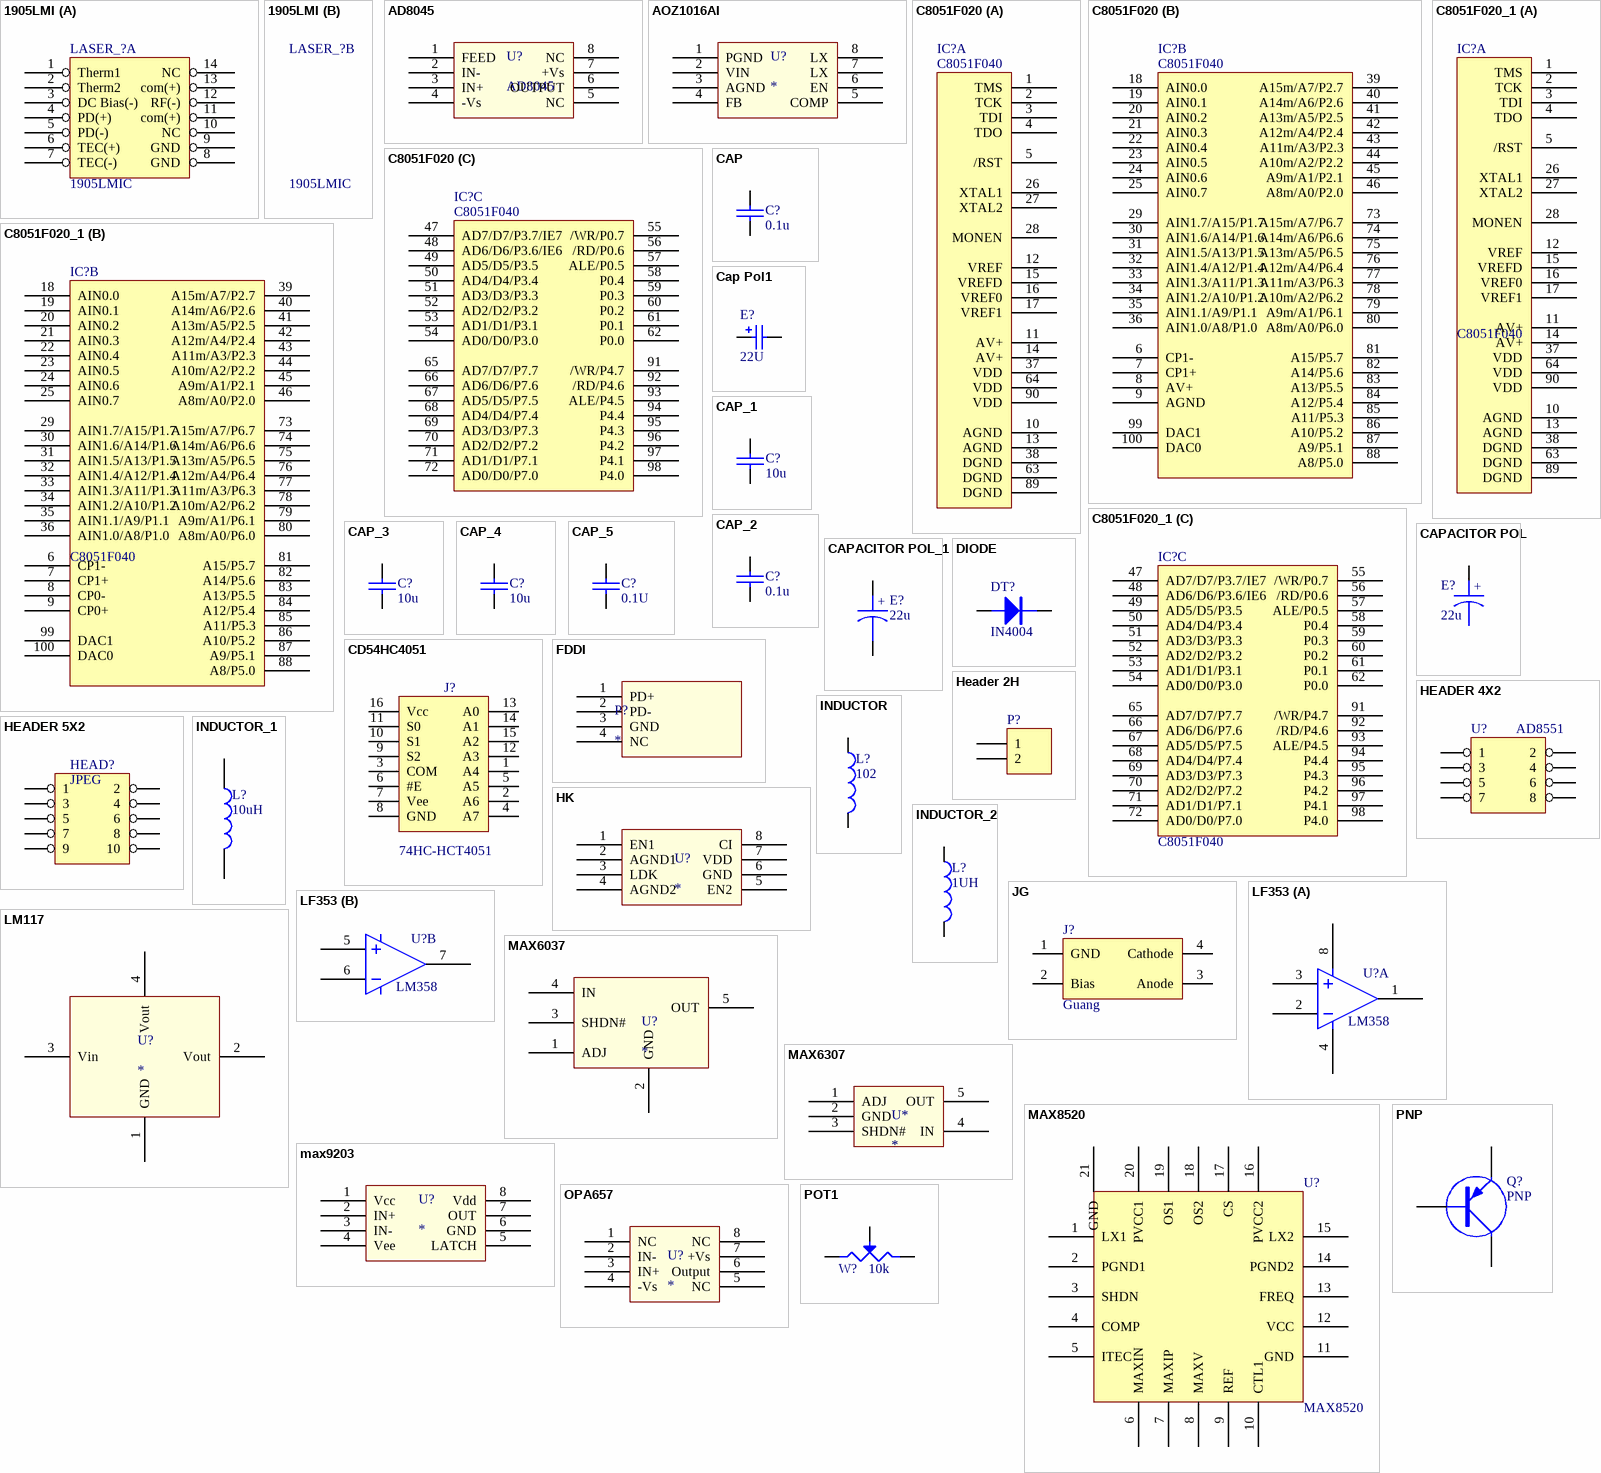
[diagram p0: symbols 1905LMI to POT1]
# Altium schematic symbol library MISC79012-5.SchLib: 47 symbols
Pins are listed as number, name and electrical type; pins without a type are passive.


## 1905LMI
designator LASER_?, comment 1905LMIC
Part Field 1: +5
footprint 1915LMM_LD
part A pins: 1 Therm1, 2 Therm2, 3 DC Bias(-), 4 PD(+), 5 PD(-), 6 TEC(+), 7 TEC(-), 8 GND, 9 GND, 10 NC, 11 com(+), 12 RF(-), 13 com(+), 14 NC

## AD8045
designator U?
pins: 1 FEED, 2 IN-, 3 IN+, 4 -Vs, 5 NC, 6 OUTPUT, 7 +Vs, 8 NC

## AOZ1016AI
designator U?
pins: 1 PGND, 2 VIN, 3 AGND, 4 FB, 5 COMP, 6 EN, 7 LX, 8 LX

## C8051F020
designator IC?, comment C8051F040
footprint TQFP100
part A pins: 1 TMS, 2 TCK, 3 TDI, 4 TDO, 5 /RST, 10 AGND, 11 AV+, 12 VREF, 13 AGND, 14 AV+, 15 VREFD, 16 VREF0, 17 VREF1, 26 XTAL1, 27 XTAL2, 28 MONEN, 37 VDD, 38 DGND, 63 DGND, 64 VDD, 89 DGND, 90 VDD
part B pins: 6 CP1-, 7 CP1+, 8 AV+, 9 AGND, 18 AIN0.0, 19 AIN0.1, 20 AIN0.2, 21 AIN0.3, 22 AIN0.4, 23 AIN0.5, 24 AIN0.6, 25 AIN0.7, 29 AIN1.7/A15/P1.7, 30 AIN1.6/A14/P1.6, 31 AIN1.5/A13/P1.5, 32 AIN1.4/A12/P1.4, 33 AIN1.3/A11/P1.3, 34 AIN1.2/A10/P1.2, 35 AIN1.1/A9/P1.1, 36 AIN1.0/A8/P1.0, 39 A15m/A7/P2.7, 40 A14m/A6/P2.6, 41 A13m/A5/P2.5, 42 A12m/A4/P2.4, 43 A11m/A3/P2.3, 44 A10m/A2/P2.2, 45 A9m/A1/P2.1, 46 A8m/A0/P2.0, 73 A15m/A7/P6.7, 74 A14m/A6/P6.6, 75 A13m/A5/P6.5, 76 A12m/A4/P6.4, 77 A11m/A3/P6.3, 78 A10m/A2/P6.2, 79 A9m/A1/P6.1, 80 A8m/A0/P6.0, 81 A15/P5.7, 82 A14/P5.6, 83 A13/P5.5, 84 A12/P5.4, 85 A11/P5.3, 86 A10/P5.2, 87 A9/P5.1, 88 A8/P5.0, 99 DAC1, 100 DAC0
part C pins: 47 AD7/D7/P3.7/IE7, 48 AD6/D6/P3.6/IE6, 49 AD5/D5/P3.5, 50 AD4/D4/P3.4, 51 AD3/D3/P3.3, 52 AD2/D2/P3.2, 53 AD1/D1/P3.1, 54 AD0/D0/P3.0, 55 /WR/P0.7, 56 /RD/P0.6, 57 ALE/P0.5, 58 P0.4, 59 P0.3, 60 P0.2, 61 P0.1, 62 P0.0, 65 AD7/D7/P7.7, 66 AD6/D6/P7.6, 67 AD5/D5/P7.5, 68 AD4/D4/P7.4, 69 AD3/D3/P7.3, 70 AD2/D2/P7.2, 71 AD1/D1/P7.1, 72 AD0/D0/P7.0, 91 /WR/P4.7, 92 /RD/P4.6, 93 ALE/P4.5, 94 P4.4, 95 P4.3, 96 P4.2, 97 P4.1, 98 P4.0
2 alternate drawings of the same symbol

## C8051F020_1
designator IC?, comment C8051F040
footprint TQFP100
part A pins: 1 TMS, 2 TCK, 3 TDI, 4 TDO, 5 /RST, 10 AGND, 11 AV+, 12 VREF, 13 AGND, 14 AV+, 15 VREFD, 16 VREF0, 17 VREF1, 26 XTAL1, 27 XTAL2, 28 MONEN, 37 VDD, 38 DGND, 63 DGND, 64 VDD, 89 DGND, 90 VDD
part B pins: 6 CP1-, 7 CP1+, 8 CP0-, 9 CP0+, 18 AIN0.0, 19 AIN0.1, 20 AIN0.2, 21 AIN0.3, 22 AIN0.4, 23 AIN0.5, 24 AIN0.6, 25 AIN0.7, 29 AIN1.7/A15/P1.7, 30 AIN1.6/A14/P1.6, 31 AIN1.5/A13/P1.5, 32 AIN1.4/A12/P1.4, 33 AIN1.3/A11/P1.3, 34 AIN1.2/A10/P1.2, 35 AIN1.1/A9/P1.1, 36 AIN1.0/A8/P1.0, 39 A15m/A7/P2.7, 40 A14m/A6/P2.6, 41 A13m/A5/P2.5, 42 A12m/A4/P2.4, 43 A11m/A3/P2.3, 44 A10m/A2/P2.2, 45 A9m/A1/P2.1, 46 A8m/A0/P2.0, 73 A15m/A7/P6.7, 74 A14m/A6/P6.6, 75 A13m/A5/P6.5, 76 A12m/A4/P6.4, 77 A11m/A3/P6.3, 78 A10m/A2/P6.2, 79 A9m/A1/P6.1, 80 A8m/A0/P6.0, 81 A15/P5.7, 82 A14/P5.6, 83 A13/P5.5, 84 A12/P5.4, 85 A11/P5.3, 86 A10/P5.2, 87 A9/P5.1, 88 A8/P5.0, 99 DAC1, 100 DAC0
part C pins: 47 AD7/D7/P3.7/IE7, 48 AD6/D6/P3.6/IE6, 49 AD5/D5/P3.5, 50 AD4/D4/P3.4, 51 AD3/D3/P3.3, 52 AD2/D2/P3.2, 53 AD1/D1/P3.1, 54 AD0/D0/P3.0, 55 /WR/P0.7, 56 /RD/P0.6, 57 ALE/P0.5, 58 P0.4, 59 P0.3, 60 P0.2, 61 P0.1, 62 P0.0, 65 AD7/D7/P7.7, 66 AD6/D6/P7.6, 67 AD5/D5/P7.5, 68 AD4/D4/P7.4, 69 AD3/D3/P7.3, 70 AD2/D2/P7.2, 71 AD1/D1/P7.1, 72 AD0/D0/P7.0, 91 /WR/P4.7, 92 /RD/P4.6, 93 ALE/P4.5, 94 P4.4, 95 P4.3, 96 P4.2, 97 P4.1, 98 P4.0
2 alternate drawings of the same symbol

## CAP
designator C?, comment 0.1u
Capacitor
footprint 0603
pins: 1, 2

## Cap Pol1
designator E?, comment 22U
Polarized Capacitor (Radial)
footprint 3528
simulation model CAP (Capacitor)
signal-integrity model Cap Pol
pins: 1, 2
1 alternate drawing of the same symbol

## CAP_1
designator C?, comment 10u
footprint 1206
pins: 1, 2

## CAP_2
designator C?, comment 0.1u
footprint 0603
pins: 1, 2

## CAP_3
designator C?, comment 10u
Capacitor
footprint 1206
pins: 1, 2

## CAP_4
designator C?, comment 10u
Capacitor
footprint 1210 (Footprint not found)
pins: 1, 2

## CAP_5
designator C?, comment 0.1U
Capacitor
footprint 0603
pins: 1, 2
2 alternate drawings of the same symbol

## CAPACITOR POL
designator E?, comment 22u
footprint 3528
pins: 1, 2

## CAPACITOR POL_1
designator E?, comment 22u
Capacitor
footprint 1210 (Footprint not found)
pins: 1, 2

## CD54HC4051
designator J?, comment 74HC-HCT4051
footprint SOIC16
pins: 1 A4, 2 A6, 3 COM, 4 A7, 5 A5, 6 #E, 7 Vee, 8 GND, 9 S2, 10 S1, 11 S0, 12 A3, 13 A0, 14 A1, 15 A2, 16 Vcc

## DIODE
designator DT?, comment IN4004
footprint DIODE04A
pins: A, K

## FDDI
designator P?
pins: 1 PD+, 2 PD-, 3 GND, 4 NC

## Header 2H
designator P?
Header, 2-Pin, Right Angle
footprint PAD2
signal-integrity model Connector
pins: 1, 2

## HEADER 4X2
designator U?, comment AD8551
footprint SO-8
pins: 1, 2, 3, 4, 5, 6, 7, 8

## HEADER 5X2
designator HEAD?, comment JPEG
footprint FKV10SN
pins: 1, 2, 3, 4, 5, 6, 7, 8, 9, 10
2 alternate drawings of the same symbol

## HK
designator U?
pins: 1 EN1, 2 AGND1, 3 LDK, 4 AGND2, 5 EN2, 6 GND, 7 VDD, 8 CI

## INDUCTOR
designator L?, comment 102
footprint INDUC3
pins: 1, 2

## INDUCTOR_1
designator L?, comment 10uH
footprint INDUC3
pins: 1, 2

## INDUCTOR_2
designator L?, comment 1UH
Text Field1: 10; Text Field2: 40
footprint 0805
pins: 1, 2
2 alternate drawings of the same symbol

## JG
designator J?, comment Guang
footprint guang (Footprint not found)
pins: 1 GND, 2 Bias, 3 Anode, 4 Cathode

## LF353
designator U?, comment LM358
footprint DIP8
footprint SO-8
part A pins: 1, 2, 3, 4, 8
part B pins: 5, 6, 7

## LM117
designator U?
pins: 1 GND, 2 Vout, 3 Vin, 4 Vout

## MAX6037
designator U?
pins: 1 ADJ, 2 GND, 3 SHDN#, 4 IN, 5 OUT

## MAX6307
designator U*
pins: 1 ADJ, 2 GND, 3 SHDN#, 4 IN, 5 OUT

## MAX8520
designator U?
footprint QFN20
pins: 1 LX1, 2 PGND1, 3 SHDN, 4 COMP, 5 ITEC, 6 MAXIN, 7 MAXIP, 8 MAXV, 9 REF, 10 CTL1, 11 GND, 12 VCC, 13 FREQ, 14 PGND2, 15 LX2, 16 PVCC2, 17 CS, 18 OS2, 19 OS1, 20 PVCC1, 21 GND

## max9203
designator U?
pins: 1 Vcc, 2 IN+, 3 IN-, 4 Vee, 5 LATCH, 6 GND, 7 OUT, 8 Vdd

## OPA657
designator U?
pins: 1 NC, 2 IN-, 3 IN+, 4 -Vs, 5 NC, 6 Output, 7 +Vs, 8 NC

## PNP
designator Q?
footprint SOT-89B
pins: 1 B, 2 C, 3 E

## POT1
designator W?, comment 10k
footprint VR4B
pins: 1, 2, 3

## POT1_1
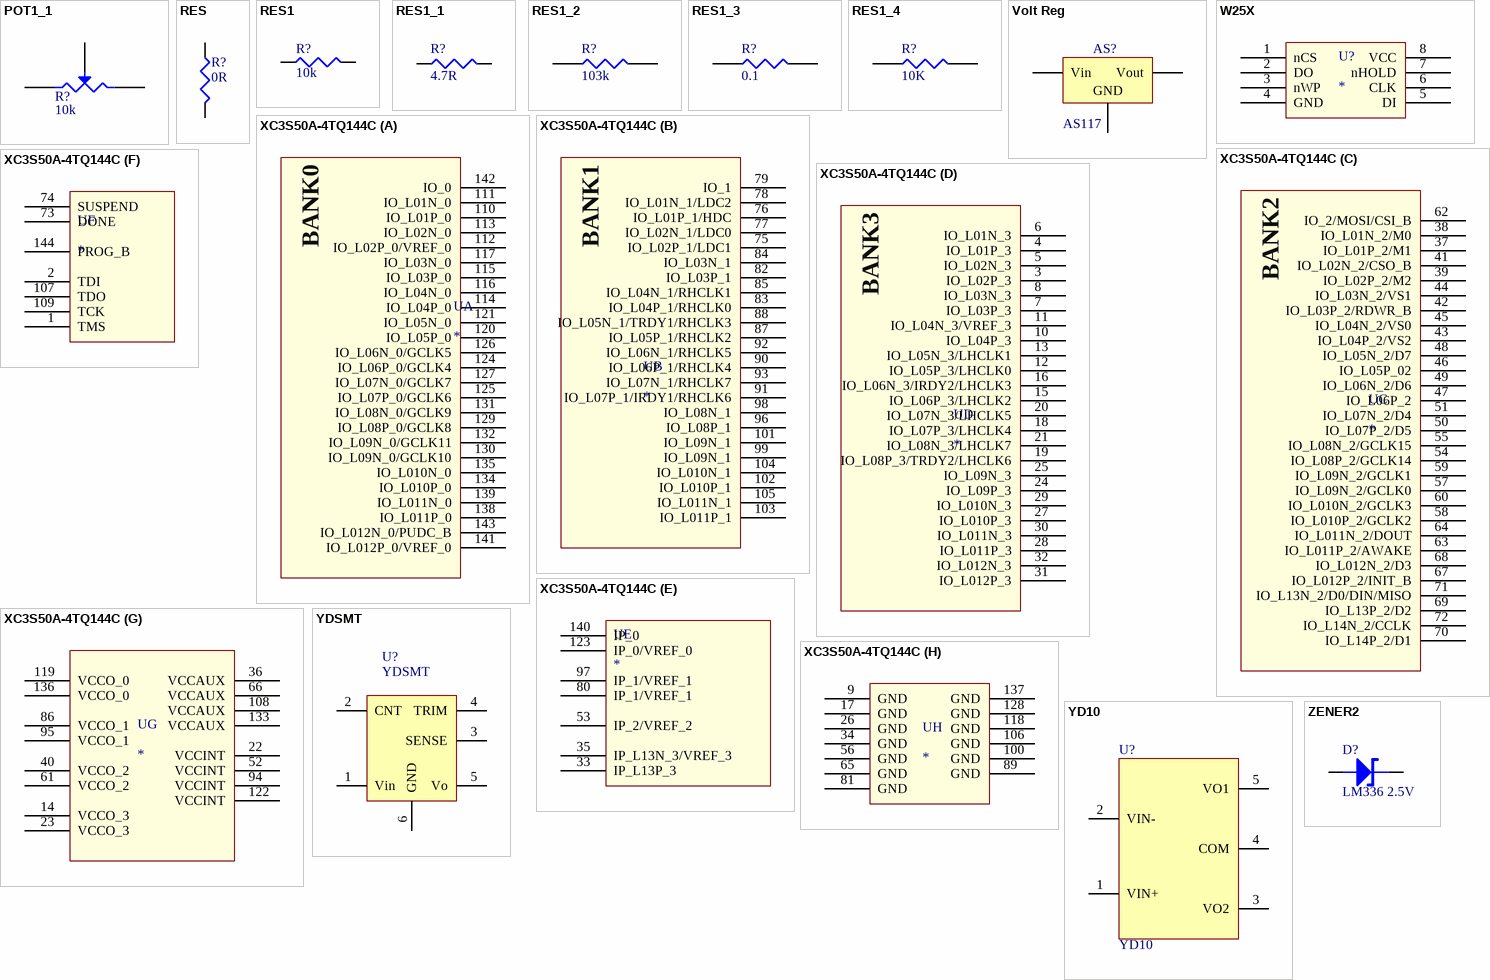
[diagram p1: symbols POT1_1 to ZENER2]
## POT1_1
designator R?, comment 10k
Potentiometer
footprint VR4B
pins: 1, 2, 3 W

## RES
designator R?, comment 0R
Resistor
footprint 0603
pins: 1, 2
2 alternate drawings of the same symbol

## RES1
designator R?, comment 10k
footprint 0603
pins: 1, 2

## RES1_1
designator R?, comment 4.7R
footprint 1206 (Footprint not found)
pins: 1, 2

## RES1_2
designator R?, comment 103k
footprint 0603
pins: 1, 2

## RES1_3
designator R?, comment 0.1
footprint 7243A
pins: 1, 2

## RES1_4
designator R?, comment 10K
footprint 0603
pins: 1, 2
2 alternate drawings of the same symbol

## Volt Reg
designator AS?, comment AS117
Voltage Regulator
footprint SOT-89
pins: 1 GND, 2 Vout, 3 Vin

## W25X
designator U?
pins: 1 nCS, 2 DO, 3 nWP, 4 GND, 5 DI, 6 CLK, 7 nHOLD, 8 VCC

## XC3S50A-4TQ144C
designator U
part A pins: 110 IO_L01P_0, 111 IO_L01N_0, 112 IO_L02P_0/VREF_0, 113 IO_L02N_0, 114 IO_L04P_0, 115 IO_L03P_0, 116 IO_L04N_0, 117 IO_L03N_0, 120 IO_L05P_0, 121 IO_L05N_0, 124 IO_L06P_0/GCLK4, 125 IO_L07P_0/GCLK6, 126 IO_L06N_0/GCLK5, 127 IO_L07N_0/GCLK7, 129 IO_L08P_0/GCLK8, 130 IO_L09N_0/GCLK10, 131 IO_L08N_0/GCLK9, 132 IO_L09N_0/GCLK11, 134 IO_L010P_0, 135 IO_L010N_0, 138 IO_L011P_0, 139 IO_L011N_0, 141 IO_L012P_0/VREF_0, 142 IO_0, 143 IO_L012N_0/PUDC_B
part B pins: 75 IO_L02P_1/LDC1, 76 IO_L01P_1/HDC, 77 IO_L02N_1/LDC0, 78 IO_L01N_1/LDC2, 79 IO_1, 82 IO_L03P_1, 83 IO_L04P_1/RHCLK0, 84 IO_L03N_1, 85 IO_L04N_1/RHCLK1, 87 IO_L05P_1/RHCLK2, 88 IO_L05N_1/TRDY1/RHCLK3, 90 IO_L06P_1/RHCLK4, 91 IO_L07P_1/IRDY1/RHCLK6, 92 IO_L06N_1/RHCLK5, 93 IO_L07N_1/RHCLK7, 96 IO_L08P_1, 98 IO_L08N_1, 99 IO_L09N_1, 101 IO_L09N_1, 102 IO_L010P_1, 103 IO_L011P_1, 104 IO_L010N_1, 105 IO_L011N_1
part C pins: 37 IO_L01P_2/M1, 38 IO_L01N_2/M0, 39 IO_L02P_2/M2, 41 IO_L02N_2/CSO_B, 42 IO_L03P_2/RDWR_B, 43 IO_L04P_2/VS2, 44 IO_L03N_2/VS1, 45 IO_L04N_2/VS0, 46 IO_L05P_02, 47 IO_L06P_2, 48 IO_L05N_2/D7, 49 IO_L06N_2/D6, 50 IO_L07P_2/D5, 51 IO_L07N_2/D4, 54 IO_L08P_2/GCLK14, 55 IO_L08N_2/GCLK15, 57 IO_L09N_2/GCLK0, 58 IO_L010P_2/GCLK2, 59 IO_L09N_2/GCLK1, 60 IO_L010N_2/GCLK3, 62 IO_2/MOSI/CSI_B, 63 IO_L011P_2/AWAKE, 64 IO_L011N_2/DOUT, 67 IO_L012P_2/INIT_B, 68 IO_L012N_2/D3, 69 IO_L13P_2/D2, 70 IO_L14P_2/D1, 71 IO_L13N_2/D0/DIN/MISO, 72 IO_L14N_2/CCLK
part D pins: 3 IO_L02P_3, 4 IO_L01P_3, 5 IO_L02N_3, 6 IO_L01N_3, 7 IO_L03P_3, 8 IO_L03N_3, 10 IO_L04P_3, 11 IO_L04N_3/VREF_3, 12 IO_L05P_3/LHCLK0, 13 IO_L05N_3/LHCLK1, 15 IO_L06P_3/LHCLK2, 16 IO_L06N_3/IRDY2/LHCLK3, 18 IO_L07P_3/LHCLK4, 19 IO_L08P_3/TRDY2/LHCLK6, 20 IO_L07N_3/LHCLK5, 21 IO_L08N_3/LHCLK7, 24 IO_L09P_3, 25 IO_L09N_3, 27 IO_L010P_3, 28 IO_L011P_3, 29 IO_L010N_3, 30 IO_L011N_3, 31 IO_L012P_3, 32 IO_L012N_3
part E pins: 33 IP_L13P_3, 35 IP_L13N_3/VREF_3, 53 IP_2/VREF_2, 80 IP_1/VREF_1, 97 IP_1/VREF_1, 123 IP_0/VREF_0, 140 IP_0
part F pins: 1 TMS, 2 TDI, 73 DONE, 74 SUSPEND, 107 TDO, 109 TCK, 144 PROG_B
part G pins: 14 VCCO_3, 22 VCCINT, 23 VCCO_3, 36 VCCAUX, 40 VCCO_2, 52 VCCINT, 61 VCCO_2, 66 VCCAUX, 86 VCCO_1, 94 VCCINT, 95 VCCO_1, 108 VCCAUX, 119 VCCO_0, 122 VCCINT, 133 VCCAUX, 136 VCCO_0
part H pins: 9 GND, 17 GND, 26 GND, 34 GND, 56 GND, 65 GND, 81 GND, 89 GND, 100 GND, 106 GND, 118 GND, 128 GND, 137 GND

## YD10
designator U?
footprint YD10
pins: 1 VIN+, 2 VIN-, 3 VO2, 4 COM, 5 VO1

## YDSMT
designator U?
footprint YDSMT1210
pins: 1 Vin, 2 CNT, 3 SENSE, 4 TRIM, 5 Vo, 6 GND

## ZENER2
designator D?, comment LM336 2.5V
footprint TO-92C
pins: A, K